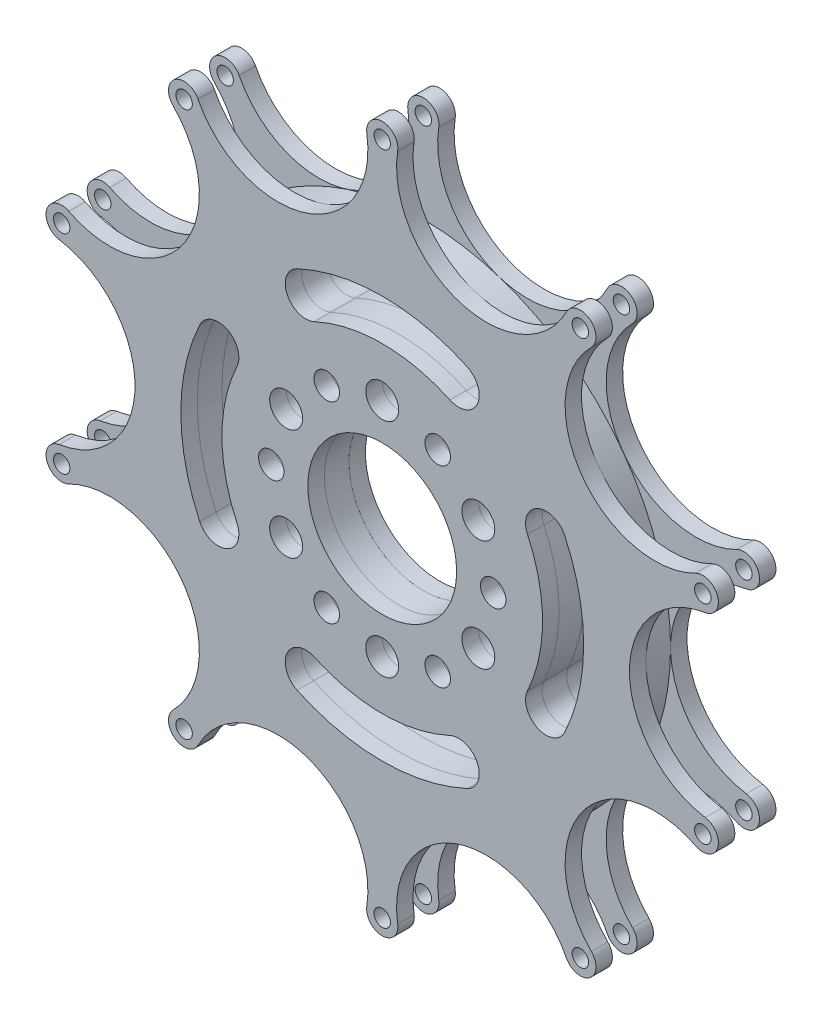
from build123d import *

# Parameters (mm, degrees)
SKETCH_1_R               = 1
EXTRUDE_2_DEPTH          = 2
SKETCH_2_R               = 30.072373867
EXTRUDE_3_DEPTH          = 3
SKETCH_3_R               = 1
EXTRUDE_4_DEPTH          = 2
SKETCH_4_R               = 1.55
SKETCH_4_R_2             = 2
CUT_EXTRUDE_1_DEPTH      = 10
CUT_EXTRUDE_3_DEPTH      = 60.679756945
CUT_EXTRUDE_3_DEPTH_BACK = 60.679756945
SKETCH_6_R               = 9.05


with BuildPart() as part:
    # 草图1 → 凸台-拉伸2 (new body)
    with BuildSketch(Plane.XY):
        with BuildLine():
            ThreePointArc((1.876607847, 40.702774516), (0, 42.9), (-1.876607847, 40.702774516))
            ThreePointArc((-1.876607847, 40.702774516), (-3.352363827, 33.283648198), (-9.292874586, 28.600527126))
            ThreePointArc((-9.292874586, 28.600527126), (-16.851518246, 28.897507045), (-22.406282948, 34.032278719))
            ThreePointArc((-22.406282948, 34.032278719), (-25.215987323, 34.706829059), (-25.442698228, 31.826193885))
            ThreePointArc((-25.442698228, 31.826193885), (-22.275756861, 24.956567009), (-24.329061519, 17.67609786))
            ThreePointArc((-24.329061519, 17.67609786), (-30.618693111, 13.473500391), (-38.130735219, 14.362609165))
            ThreePointArc((-38.130735219, 14.362609165), (-40.800324549, 13.256829059), (-39.290542652, 10.793088922))
            ThreePointArc((-39.290542652, 10.793088922), (-32.690567898, 7.096925465), (-30.072373867, 0))
            ThreePointArc((-30.072373867, 0), (-32.690567898, -7.096925465), (-39.290542652, -10.793088922))
            ThreePointArc((-39.290542652, -10.793088922), (-40.800324549, -13.256829059), (-38.130735219, -14.362609165))
            ThreePointArc((-38.130735219, -14.362609165), (-30.618693111, -13.473500391), (-24.329061519, -17.67609786))
            ThreePointArc((-24.329061519, -17.67609786), (-22.275756861, -24.956567009), (-25.442698228, -31.826193885))
            ThreePointArc((-25.442698228, -31.826193885), (-25.215987323, -34.706829059), (-22.406282948, -34.032278719))
            ThreePointArc((-22.406282948, -34.032278719), (-16.851518246, -28.897507045), (-9.292874586, -28.600527126))
            ThreePointArc((-9.292874586, -28.600527126), (-3.352363827, -33.283648198), (-1.876607847, -40.702774516))
            ThreePointArc((-1.876607847, -40.702774516), (0, -42.9), (1.876607847, -40.702774516))
            ThreePointArc((1.876607847, -40.702774516), (3.352363827, -33.283648198), (9.292874586, -28.600527126))
            ThreePointArc((9.292874586, -28.600527126), (16.851518246, -28.897507045), (22.406282948, -34.032278719))
            ThreePointArc((22.406282948, -34.032278719), (25.215987323, -34.706829059), (25.442698228, -31.826193885))
            ThreePointArc((25.442698228, -31.826193885), (22.275756861, -24.956567009), (24.329061519, -17.67609786))
            ThreePointArc((24.329061519, -17.67609786), (30.618693111, -13.473500391), (38.130735219, -14.362609165))
            ThreePointArc((38.130735219, -14.362609165), (40.800324549, -13.256829059), (39.290542652, -10.793088922))
            ThreePointArc((39.290542652, -10.793088922), (32.690567898, -7.096925465), (30.072373867, 0))
            ThreePointArc((30.072373867, 0), (32.690567898, 7.096925465), (39.290542652, 10.793088922))
            ThreePointArc((39.290542652, 10.793088922), (40.800324549, 13.256829059), (38.130735219, 14.362609165))
            ThreePointArc((38.130735219, 14.362609165), (30.618693111, 13.473500391), (24.329061519, 17.67609786))
            ThreePointArc((24.329061519, 17.67609786), (22.275756861, 24.956567009), (25.442698228, 31.826193885))
            ThreePointArc((25.442698228, 31.826193885), (25.215987323, 34.706829059), (22.406282948, 34.032278719))
            ThreePointArc((22.406282948, 34.032278719), (16.851518246, 28.897507045), (9.292874586, 28.600527126))
            ThreePointArc((9.292874586, 28.600527126), (3.352363827, 33.283648198), (1.876607847, 40.702774516))
        make_face()
        with Locations((0, 41)):
            Circle(SKETCH_1_R, mode=Mode.SUBTRACT)
        with Locations((24.099195344, 33.169696769)):
            Circle(SKETCH_1_R, mode=Mode.SUBTRACT)
        with Locations((38.993317168, 12.669696769)):
            Circle(SKETCH_1_R, mode=Mode.SUBTRACT)
        with Locations((38.993317168, -12.669696769)):
            Circle(SKETCH_1_R, mode=Mode.SUBTRACT)
        with Locations((24.099195344, -33.169696769)):
            Circle(SKETCH_1_R, mode=Mode.SUBTRACT)
        with Locations((0, -41)):
            Circle(SKETCH_1_R, mode=Mode.SUBTRACT)
        with Locations((-24.099195344, -33.169696769)):
            Circle(SKETCH_1_R, mode=Mode.SUBTRACT)
        with Locations((-38.993317168, -12.669696769)):
            Circle(SKETCH_1_R, mode=Mode.SUBTRACT)
        with Locations((-38.993317168, 12.669696769)):
            Circle(SKETCH_1_R, mode=Mode.SUBTRACT)
        with Locations((-24.099195344, 33.169696769)):
            Circle(SKETCH_1_R, mode=Mode.SUBTRACT)
    extrude(amount=EXTRUDE_2_DEPTH)


with BuildPart() as body_2:
    # 草图2 → 凸台-拉伸3 (new body)
    with BuildSketch(Plane.XY.offset(2)):
        Circle(SKETCH_2_R)
    extrude(amount=EXTRUDE_3_DEPTH)


with BuildPart() as body_3:
    # 草图3 → 凸台-拉伸4 (new body)
    with BuildSketch(Plane.XY.offset(5)):
        with BuildLine():
            ThreePointArc((-22.406282948, 34.032278719), (-9.292874586, 28.600527126), (-1.876607847, 40.702774516))
            ThreePointArc((-1.876607847, 40.702774516), (0, 42.9), (1.876607847, 40.702774516))
            ThreePointArc((1.876607847, 40.702774516), (9.292874586, 28.600527126), (22.406282948, 34.032278719))
            ThreePointArc((22.406282948, 34.032278719), (25.215987323, 34.706829059), (25.442698228, 31.826193885))
            ThreePointArc((25.442698228, 31.826193885), (24.329061519, 17.67609786), (38.130735219, 14.362609165))
            ThreePointArc((38.130735219, 14.362609165), (40.800324549, 13.256829059), (39.290542652, 10.793088922))
            ThreePointArc((39.290542652, 10.793088922), (30.072373867, 0), (39.290542652, -10.793088922))
            ThreePointArc((39.290542652, -10.793088922), (40.800324549, -13.256829059), (38.130735219, -14.362609165))
            ThreePointArc((38.130735219, -14.362609165), (24.329061519, -17.67609786), (25.442698228, -31.826193885))
            ThreePointArc((25.442698228, -31.826193885), (25.215987323, -34.706829059), (22.406282948, -34.032278719))
            ThreePointArc((22.406282948, -34.032278719), (9.292874586, -28.600527126), (1.876607847, -40.702774516))
            ThreePointArc((1.876607847, -40.702774516), (0, -42.9), (-1.876607847, -40.702774516))
            ThreePointArc((-1.876607847, -40.702774516), (-9.292874586, -28.600527126), (-22.406282948, -34.032278719))
            ThreePointArc((-22.406282948, -34.032278719), (-25.215987323, -34.706829059), (-25.442698228, -31.826193885))
            ThreePointArc((-25.442698228, -31.826193885), (-24.329061519, -17.67609786), (-38.130735219, -14.362609165))
            ThreePointArc((-38.130735219, -14.362609165), (-40.800324549, -13.256829059), (-39.290542652, -10.793088922))
            ThreePointArc((-39.290542652, -10.793088922), (-30.072373867, 0), (-39.290542652, 10.793088922))
            ThreePointArc((-39.290542652, 10.793088922), (-40.800324549, 13.256829059), (-38.130735219, 14.362609165))
            ThreePointArc((-38.130735219, 14.362609165), (-24.329061519, 17.67609786), (-25.442698228, 31.826193885))
            ThreePointArc((-25.442698228, 31.826193885), (-25.215987323, 34.706829059), (-22.406282948, 34.032278719))
        make_face()
        with Locations((-38.993317168, -12.669696769)):
            Circle(SKETCH_3_R, mode=Mode.SUBTRACT)
        with Locations((-38.993317168, 12.669696769)):
            Circle(SKETCH_3_R, mode=Mode.SUBTRACT)
        with Locations((-24.099195344, 33.169696769)):
            Circle(SKETCH_3_R, mode=Mode.SUBTRACT)
        with Locations((0, 41)):
            Circle(SKETCH_3_R, mode=Mode.SUBTRACT)
        with Locations((24.099195344, 33.169696769)):
            Circle(SKETCH_3_R, mode=Mode.SUBTRACT)
        with Locations((38.993317168, 12.669696769)):
            Circle(SKETCH_3_R, mode=Mode.SUBTRACT)
        with Locations((38.993317168, -12.669696769)):
            Circle(SKETCH_3_R, mode=Mode.SUBTRACT)
        with Locations((24.099195344, -33.169696769)):
            Circle(SKETCH_3_R, mode=Mode.SUBTRACT)
        with Locations((0, -41)):
            Circle(SKETCH_3_R, mode=Mode.SUBTRACT)
        with Locations((-24.099195344, -33.169696769)):
            Circle(SKETCH_3_R, mode=Mode.SUBTRACT)
    extrude(amount=EXTRUDE_4_DEPTH)


with BuildPart() as cut_extrude_1_tool:
    # 草图4 → 切除-拉伸1 (new body)
    with BuildSketch(Plane.XY.offset(7)):
        with Locations((13.5, 0)):
            Circle(SKETCH_4_R)
        with Locations((11.691342951, 6.75)):
            Circle(SKETCH_4_R_2)
        with Locations((11.691342951, -6.75)):
            Circle(SKETCH_4_R_2)
        with Locations((6.75, -11.691342951)):
            Circle(SKETCH_4_R)
        with Locations((0, -13.5)):
            Circle(SKETCH_4_R_2)
        with Locations((-6.75, -11.691342951)):
            Circle(SKETCH_4_R)
        with Locations((-11.691342951, -6.75)):
            Circle(SKETCH_4_R_2)
        with Locations((-13.5, 0)):
            Circle(SKETCH_4_R)
        with Locations((-11.691342951, 6.75)):
            Circle(SKETCH_4_R_2)
        with Locations((-6.75, 11.691342951)):
            Circle(SKETCH_4_R)
        with Locations((0, 13.5)):
            Circle(SKETCH_4_R_2)
        with Locations((6.75, 11.691342951)):
            Circle(SKETCH_4_R)
        with BuildLine():
            ThreePointArc((22.204540782, -10.354147413), (24.5, 0), (22.204540782, 10.354147413))
            ThreePointArc((22.204540782, 10.354147413), (18.88222566, 11.563371226), (17.673001847, 8.241056104))
            ThreePointArc((17.673001847, 8.241056104), (19.5, 0), (17.673001847, -8.241056104))
            ThreePointArc((17.673001847, -8.241056104), (18.88222566, -11.563371226), (22.204540782, -10.354147413))
        make_face()
        with BuildLine():
            ThreePointArc((-10.354147413, -22.204540782), (0, -24.5), (10.354147413, -22.204540782))
            ThreePointArc((10.354147413, -22.204540782), (11.563371226, -18.88222566), (8.241056104, -17.673001847))
            ThreePointArc((8.241056104, -17.673001847), (0, -19.5), (-8.241056104, -17.673001847))
            ThreePointArc((-8.241056104, -17.673001847), (-11.563371226, -18.88222566), (-10.354147413, -22.204540782))
        make_face()
        with BuildLine():
            ThreePointArc((-22.204540782, 10.354147413), (-24.5, 0), (-22.204540782, -10.354147413))
            ThreePointArc((-22.204540782, -10.354147413), (-18.88222566, -11.563371226), (-17.673001847, -8.241056104))
            ThreePointArc((-17.673001847, -8.241056104), (-19.5, 0), (-17.673001847, 8.241056104))
            ThreePointArc((-17.673001847, 8.241056104), (-18.88222566, 11.563371226), (-22.204540782, 10.354147413))
        make_face()
        with BuildLine():
            ThreePointArc((10.354147413, 22.204540782), (0, 24.5), (-10.354147413, 22.204540782))
            ThreePointArc((-10.354147413, 22.204540782), (-11.563371226, 18.88222566), (-8.241056104, 17.673001847))
            ThreePointArc((-8.241056104, 17.673001847), (0, 19.5), (8.241056104, 17.673001847))
            ThreePointArc((8.241056104, 17.673001847), (11.563371226, 18.88222566), (10.354147413, 22.204540782))
        make_face()
    extrude(amount=-CUT_EXTRUDE_1_DEPTH)


with BuildPart() as part_1:
    add(part.part)

    # 切除-拉伸1: cut by cut_extrude_1_tool
    add(cut_extrude_1_tool.part, mode=Mode.SUBTRACT)


with BuildPart() as body_2_1:
    add(body_2.part)

    # 切除-拉伸1: cut by cut_extrude_1_tool
    add(cut_extrude_1_tool.part, mode=Mode.SUBTRACT)


with BuildPart() as body_3_1:
    add(body_3.part)

    # 切除-拉伸1: cut by cut_extrude_1_tool
    add(cut_extrude_1_tool.part, mode=Mode.SUBTRACT)


with BuildPart() as cut_extrude_3_tool:
    # 草图6 → 切除-拉伸3 (new, two sides: drawn at the far end of the back side and taken through both)
    with BuildSketch(Plane.XY.offset(7).offset(-CUT_EXTRUDE_3_DEPTH_BACK)):
        Circle(SKETCH_6_R)
    extrude(amount=CUT_EXTRUDE_3_DEPTH + CUT_EXTRUDE_3_DEPTH_BACK)


with BuildPart() as part_2:
    add(part_1.part)

    # 切除-拉伸3: cut by cut_extrude_3_tool
    add(cut_extrude_3_tool.part, mode=Mode.SUBTRACT)


with BuildPart() as body_2_2:
    add(body_2_1.part)

    # 切除-拉伸3: cut by cut_extrude_3_tool
    add(cut_extrude_3_tool.part, mode=Mode.SUBTRACT)


with BuildPart() as body_3_2:
    add(body_3_1.part)

    # 切除-拉伸3: cut by cut_extrude_3_tool
    add(cut_extrude_3_tool.part, mode=Mode.SUBTRACT)


solid = Compound([part_2.part, body_2_2.part, body_3_2.part])
